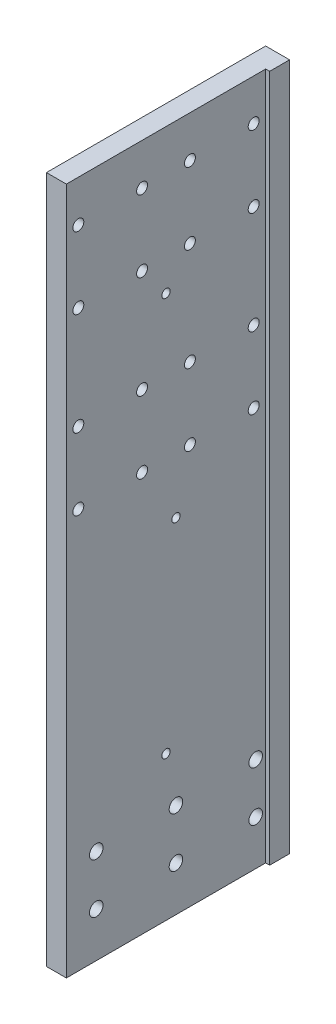
from build123d import *

# Parameters (mm, degrees)
SKETCH_1_W                   = 110
SKETCH_1_H                   = 345
EXTRUDE_1_DEPTH              = 6
SKETCH_2_W                   = 100
SKETCH_2_H                   = 345
CUT_EXTRUDE_1_DEPTH          = 2
HOLE_WIZARD_M5_1_D           = 5.5
HOLE_WIZARD_M5_1_CBORE_D     = 10
HOLE_WIZARD_M5_1_CBORE_DEPTH = 5.4
HOLE_WIZARD_M8_1_D           = 6.8
HOLE_WIZARD_M5_1_2_D         = 4.2
HOLE_WIZARD_M6_1_D           = 5
HOLE_WIZARD_M6_1_DEPTH       = 15
HOLE_WIZARD_M6_1_TIP         = 1.502151548


with BuildPart() as part:
    # 草图1 → 凸台-拉伸1 (new, symmetric)
    with BuildSketch(Plane(origin=(0, 0, 0), x_dir=(0, 0, -1), z_dir=(1, 0, 0))):
        Rectangle(SKETCH_1_W, SKETCH_1_H)
    extrude(amount=EXTRUDE_1_DEPTH, both=True)

    # 草图2 → 切除-拉伸1 (cut)
    with BuildSketch(Plane(origin=(6, 0, 0), x_dir=(0, 0, -1), z_dir=(1, 0, 0))):
        with Locations((-5, 0)):
            Rectangle(SKETCH_2_W, SKETCH_2_H)
    extrude(amount=-CUT_EXTRUDE_1_DEPTH, mode=Mode.SUBTRACT)

    # Hole Wizard M5 _1 (through all)
    with Locations(Plane.ZY.offset(6)):
        with Locations((-39, 151.75000402), (-7, 151.75000402), (17, 151.75000402), (49, 151.75000402), (49, 115.75000402), (17, 115.75000402), (-7, 115.75000402), (-39, 115.75000402), (-39, 64.250000001), (-7, 64.250000001), (17, 64.250000001), (49, 64.250000001), (-39, 28.250000001), (-7, 28.250000001), (17, 28.250000001), (49, 28.250000001)):
            CounterBoreHole(HOLE_WIZARD_M5_1_D / 2, HOLE_WIZARD_M5_1_CBORE_D / 2, HOLE_WIZARD_M5_1_CBORE_DEPTH)

    # M8 螺纹孔1 (through all)
    with Locations(Plane.ZY.offset(6)):
        with Locations((-40, -125), (-40, -150), (0, -125), (0, -150), (40, -125), (40, -150)):
            Hole(HOLE_WIZARD_M8_1_D / 2)

    # Hole Wizard M5 _1 2 (through all)
    with Locations(Plane.ZY.offset(6)):
        with Locations((0, 0), (5, 100), (5, 185), (5, -100)):
            Hole(HOLE_WIZARD_M5_1_2_D / 2)

    # M6 螺纹孔1
    with Locations(Plane(origin=(0, 0, -55), x_dir=(-1, 0, 0), z_dir=(0, 0, -1))):
        with Locations((0, 157.5), (0, 120), (0, 82.5), (0, 45), (0, 7.5)):
            Hole(HOLE_WIZARD_M6_1_D / 2, depth=HOLE_WIZARD_M6_1_DEPTH)
            with Locations((0, 0, -(HOLE_WIZARD_M6_1_DEPTH + HOLE_WIZARD_M6_1_TIP / 2))):  # 118° drill point
                Cone(0, HOLE_WIZARD_M6_1_D / 2, HOLE_WIZARD_M6_1_TIP, mode=Mode.SUBTRACT)


solid = part.part
